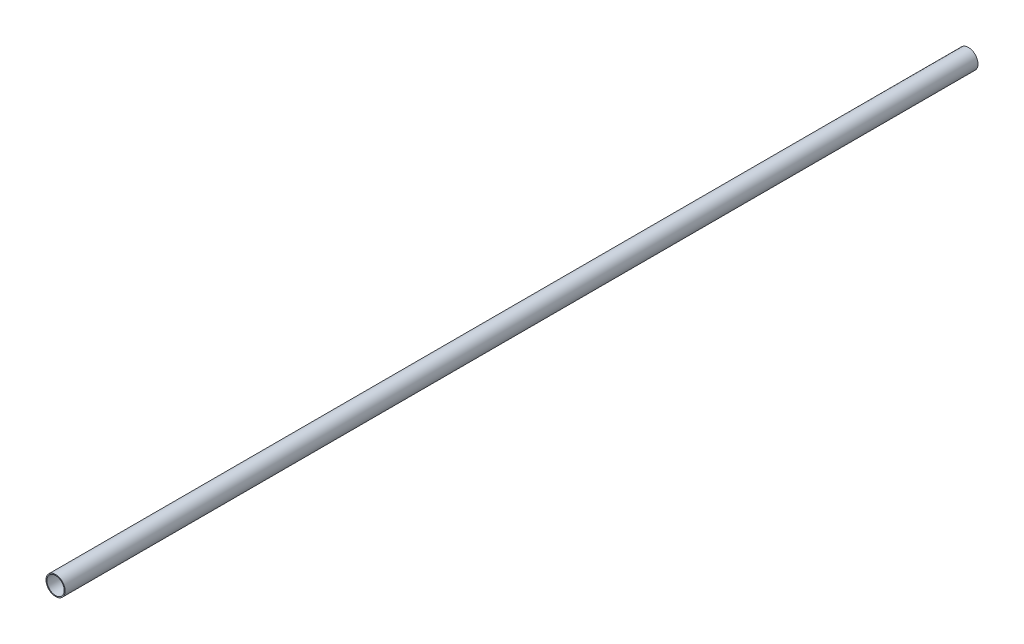
from build123d import *

# Parameters (mm, degrees)
SKETCH1_R           = 21
SKETCH1_R_2         = 19
BOSS_EXTRUDE1_DEPTH = 2000


with BuildPart() as part:
    # Sketch1 → Boss-Extrude1 (new body)
    with BuildSketch(Plane.XY):
        Circle(SKETCH1_R)
        Circle(SKETCH1_R_2, mode=Mode.SUBTRACT)
    extrude(amount=BOSS_EXTRUDE1_DEPTH)


solid = part.part
